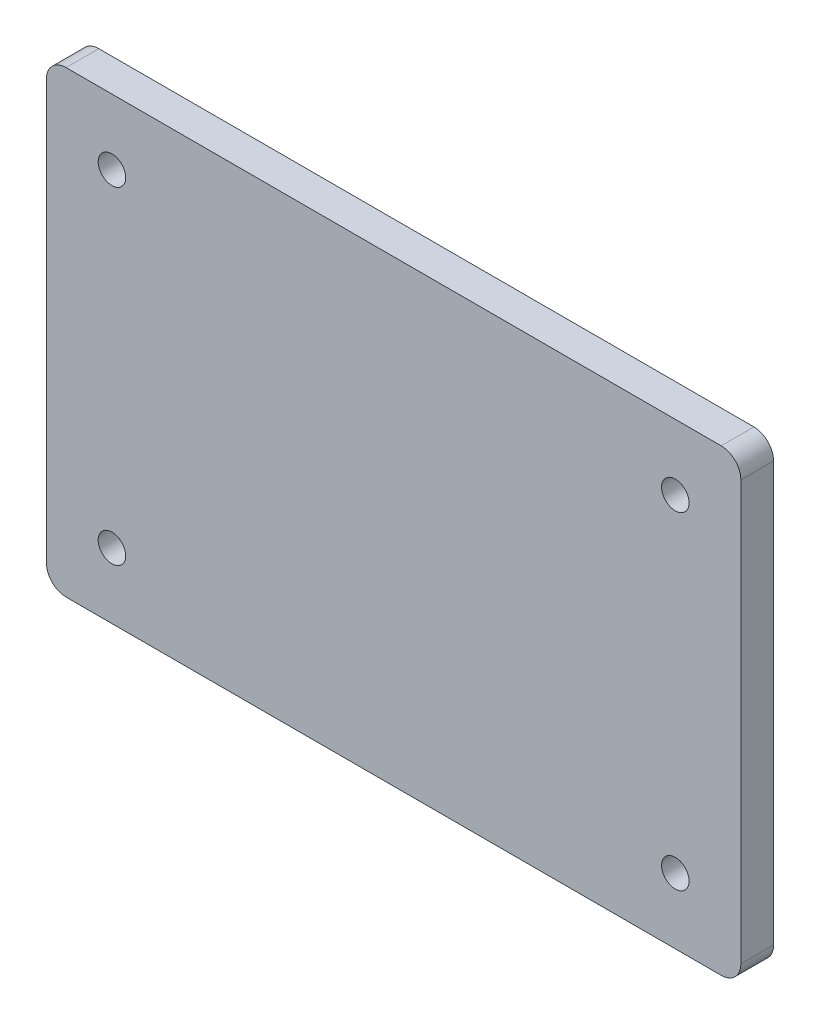
from build123d import *

# Parameters (mm, degrees)
SKETCH_1_W          = 106
SKETCH_1_H          = 70
EXTRUDE_1_DEPTH     = 2.5
SKETCH_2_R          = 2.1
CUT_EXTRUDE_1_DEPTH = 64.710281745
FILLET_1_R          = 3


with BuildPart() as part:
    # 草图1 → 凸台-拉伸1 (new, symmetric)
    with BuildSketch(Plane.XY):
        Rectangle(SKETCH_1_W, SKETCH_1_H)
    extrude(amount=EXTRUDE_1_DEPTH, both=True)

    # 草图2 → 切除-拉伸1 (cut, through all)
    with BuildSketch(Plane.XY.offset(2.5)):
        with Locations((-43, 25)):
            Circle(SKETCH_2_R)
        with Locations(Location((43, 25, 0), (0, 0, 180))):
            Circle(SKETCH_2_R)
        with Locations((43, -25)):
            Circle(SKETCH_2_R)
        with Locations(Location((-43, -25, 0), (0, 0, 180))):
            Circle(SKETCH_2_R)
    extrude(amount=-CUT_EXTRUDE_1_DEPTH, mode=Mode.SUBTRACT)

    # 圆角1
    fillet_1_edges = [part.edges().sort_by_distance(p)[0] for p in [
        (53, -35, 0),
        (-53, -35, 0),
        (-53, 35, 0),
        (53, 35, 0),
    ]]
    fillet(fillet_1_edges, radius=FILLET_1_R)


solid = part.part
